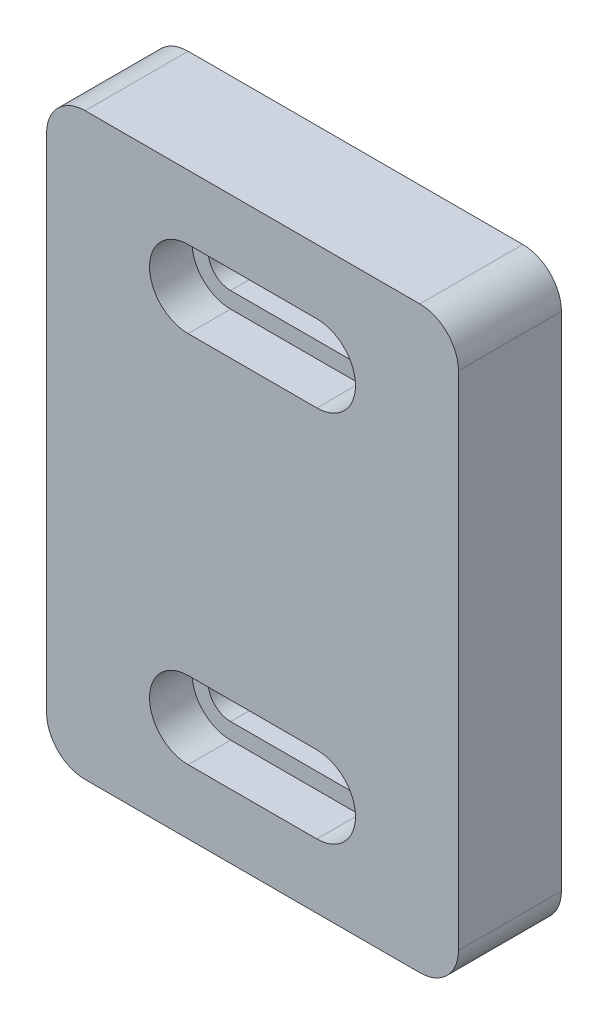
SolidWorks part; units mm, degrees
ref_plane "Front Plane" through (0, 0, 0) normal (0, 0, 1) x (1, 0, 0)
ref_plane "Top Plane" through (0, 0, 0) normal (0, 1, 0) x (1, 0, 0)
ref_plane "Right Plane" through (0, 0, 0) normal (1, 0, 0) x (0, 0, -1)
sketch "Sketch1" plane through (0, 0, 0) normal (0, 0, 1) x (1, 0, 0)
  line L1 (16, -22.5) -> (-16, -22.5)
  line L2 (16, -22.5) -> (16, 22.5)
  line L3 (16, 22.5) -> (-16, 22.5)
  line L4 (-16, -22.5) -> (-16, 22.5)
  line L5 (16, -22.5) -> (-16, 22.5) construction
  line L6 (16, 22.5) -> (-16, -22.5) construction
  point P0 (0, 0)
  dimension "D1" = 32
  dimension "D2" = 45
extrude "Boss-Extrude1" add sketch "Sketch1" along normal blind 8
fillet "Fillet1" radius 3 4 edges at (-16, -22.5, 4) (16, -22.5, 4) (16, 22.5, 4) (-16, 22.5, 4)
sketch "Sketch2" plane through (0, 0, 8) normal (0, 0, 1) x (1, 0, 0)
  line L0 (-5, 14.5) -> (5, 14.5) construction
  line L1 (-5, 16.25) -> (5, 16.25)
  line L2 (-5, 12.75) -> (5, 12.75)
  line L3 (-5, -14.5) -> (5, -14.5) construction
  line L4 (-5, -12.75) -> (5, -12.75)
  line L5 (-5, -16.25) -> (5, -16.25)
  arc A0 (-5, 16.25) -> (-5, 12.75) centre (-5, 14.5) ccw
  arc A1 (5, 12.75) -> (5, 16.25) centre (5, 14.5) ccw
  arc A2 (-5, -12.75) -> (-5, -16.25) centre (-5, -14.5) ccw
  arc A3 (5, -16.25) -> (5, -12.75) centre (5, -14.5) ccw
  point P2 (0, 14.5)
  point P7 (0, -14.5)
  dimension "D1" = 1.75
  dimension "D2" = 1.75
  dimension "D3" = 29
  dimension "D4" = 14.5
  dimension "D5" = 10
  dimension "D6" = 10
extrude "Cut-Extrude1" cut sketch "Sketch2" against normal through all
sketch "Sketch3" plane through (0, 0, 8) normal (0, 0, 1) x (1, 0, 0)
  line L0 (-5, 14.5) -> (5, 14.5) construction
  line L1 (-5, 17.5) -> (5, 17.5)
  line L2 (-5, 11.5) -> (5, 11.5)
  line L3 (-5, -14.5) -> (5, -14.5) construction
  line L4 (-5, -11.5) -> (5, -11.5)
  line L5 (-5, -17.5) -> (5, -17.5)
  arc A0 (-5, 17.5) -> (-5, 11.5) centre (-5, 14.5) ccw
  arc A1 (5, 11.5) -> (5, 17.5) centre (5, 14.5) ccw
  arc A2 (-5, -11.5) -> (-5, -17.5) centre (-5, -14.5) ccw
  arc A3 (5, -17.5) -> (5, -11.5) centre (5, -14.5) ccw
  point P3 (0, 14.5)
  point P8 (0, -14.5)
  dimension "D1" = 3
  dimension "D2" = 3
  dimension "D3" = 3
extrude "Cut-Extrude2" cut sketch "Sketch3" against normal blind 3.3
